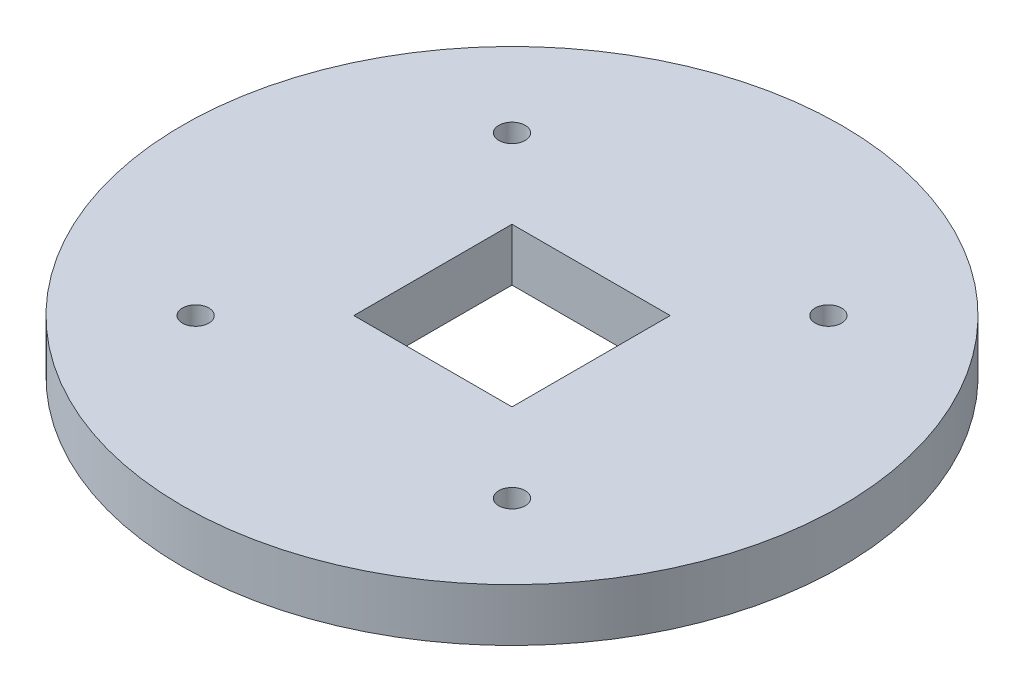
from build123d import *

# Parameters (mm, degrees)
SKETCH1_R           = 12.5
SKETCH1_R_2         = 0.5
SKETCH1_W           = 6
SKETCH1_H           = 6
BOSS_EXTRUDE1_DEPTH = 2


with BuildPart() as part:
    # Sketch1 → Boss-Extrude1 (new body)
    with BuildSketch(Plane(origin=(0, 0, 0), x_dir=(1, 0, 0), z_dir=(0, 1, 0))):
        with Locations(Location((0, 0, 0), (0, 0, 270))):
            Circle(SKETCH1_R)
        with Locations(Location((-6, 6, 0), (0, 0, 270))):
            Circle(SKETCH1_R_2, mode=Mode.SUBTRACT)
        with Locations(Location((6, 6, 0), (0, 0, 270))):
            Circle(SKETCH1_R_2, mode=Mode.SUBTRACT)
        with Locations(Location((-6, -6, 0), (0, 0, 270))):
            Circle(SKETCH1_R_2, mode=Mode.SUBTRACT)
        with Locations(Location((6, -6, 0), (0, 0, 270))):
            Circle(SKETCH1_R_2, mode=Mode.SUBTRACT)
        Rectangle(SKETCH1_W, SKETCH1_H, mode=Mode.SUBTRACT)
    extrude(amount=BOSS_EXTRUDE1_DEPTH)


solid = part.part
